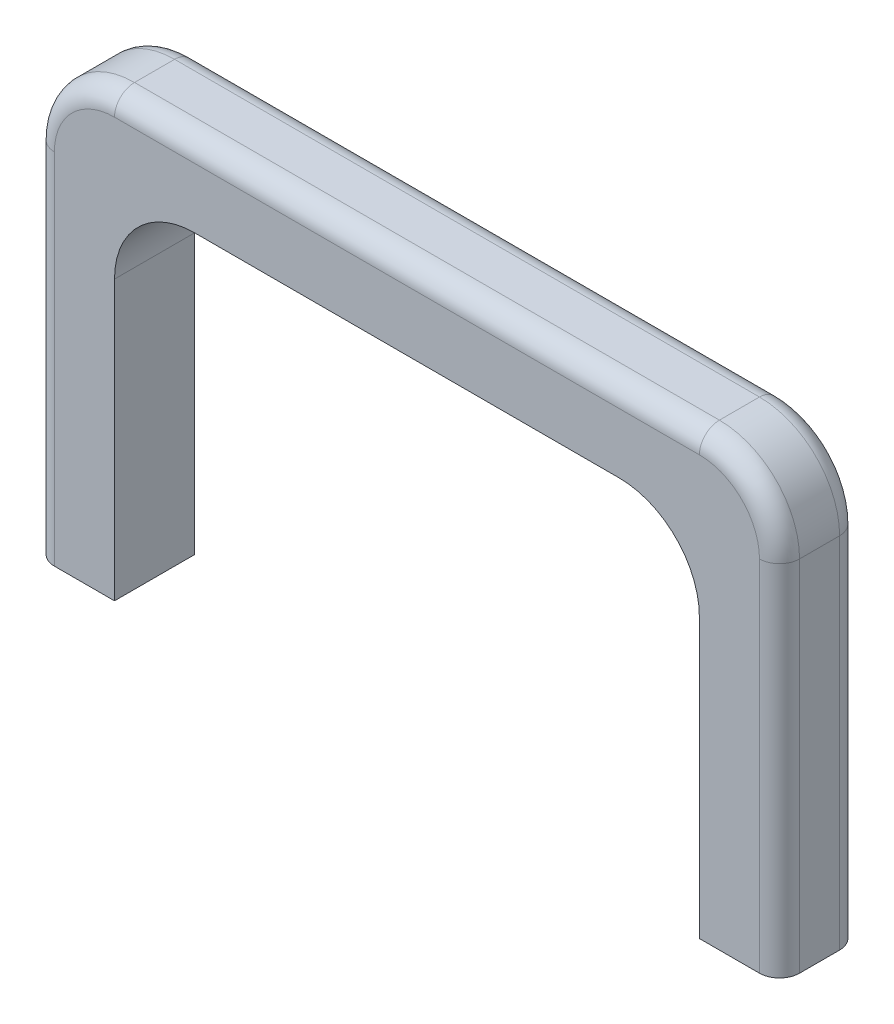
SolidWorks part; units mm, degrees
ref_plane "Front Plane" through (0, 0, 0) normal (0, 0, 1) x (1, 0, 0)
ref_plane "Top Plane" through (0, 0, 0) normal (0, 1, 0) x (1, 0, 0)
ref_plane "Right Plane" through (0, 0, 0) normal (1, 0, 0) x (0, 0, -1)
sketch "Sketch1" plane through (0, 0, 0) normal (0, 0, 1) x (1, 0, 0)
  line L2 (0, 0) -> (0, 8.9545)
  line L3 (0, 8.9545) -> (14.5968, 8.9545)
  line L4 (14.5968, 0) -> (14.5968, 8.9545)
extrude "Extrude-Thin1" add sketch "Sketch1" along normal blind 2 thin thin type one direction wall 2
fillet "Fillet1" radius 2 4 edges at (14.5968, 8.9545, 1) (0, 8.9545, 1) (16.5968, 10.9545, 1) (-2, 10.9545, 1)
fillet "Fillet2" radius 0.5 10 edges at (16.5968, 4.4772, 0) (16.011, 10.3687, 0) (-2, 4.4772, 0) (-1.4142, 10.3687, 0) (16.5968, 4.4772, 2) (16.011, 10.3687, 2) (-2, 4.4772, 2) (-1.4142, 10.3687, 2) (7.2984, 10.9545, 0) (7.2984, 10.9545, 2)
